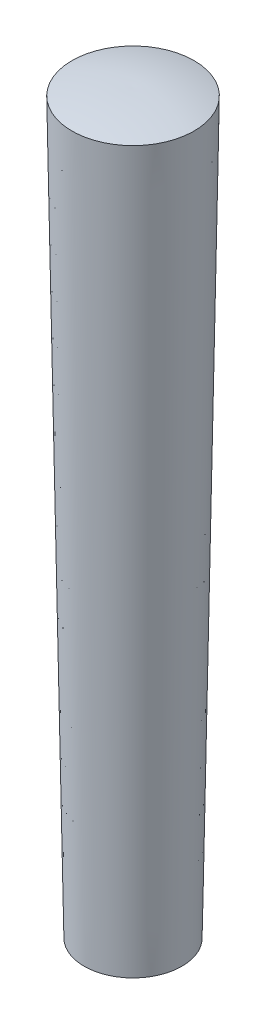
from build123d import *

# Parameters (mm, degrees)
SCALE_1_SCALE = 1.875


with BuildPart() as part:
    # Sketch1 → Revolve1 (revolve)
    with BuildSketch(Plane.XY, mode=Mode.PRIVATE) as revolve1_sk:
        with BuildLine():
            Line((-3.616060596, 37.025813588), (-2.896044906, -6.175127807))
            ThreePointArc((-2.896044906, -6.175127807), (-1.466498616, -6.530498208), (0, -6.669323733))
            Line((0, -6.669323733), (0, 0))
            Line((0, 0), (0, 30.062177826))
            Line((0, 30.062177826), (0, 37.476603875))
            ThreePointArc((0, 37.476603875), (-1.8244983, 37.383308497), (-3.616060596, 37.025813588))
        make_face()
    revolve(revolve1_sk.sketch.rotate(Axis((0, 0, 0), (0, 1, 0)), 270), axis=Axis((0, 0, 0), (0, 1, 0)))


with BuildPart() as part_1:
    # Scale 1: scaled about (0, 17.046427659, 0)
    add(part.part.scale(SCALE_1_SCALE).moved(Location((0, -14.915624202, 0))))


solid = part_1.part
